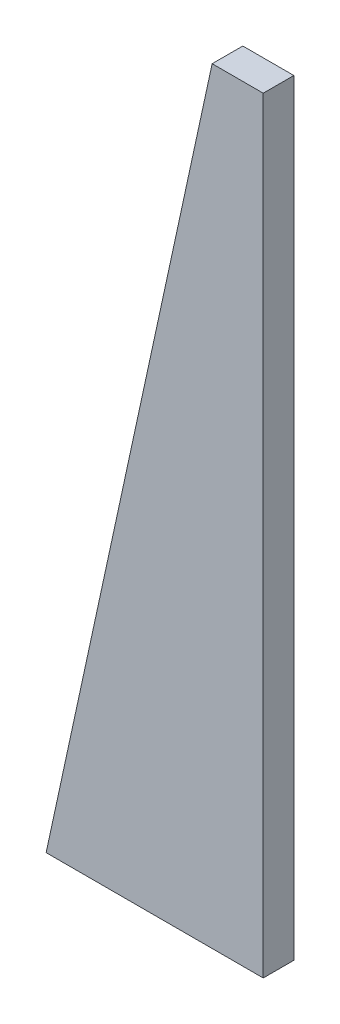
SolidWorks part; units mm, degrees
material "普通碳钢"
ref_plane "Front Plane" through (0, 0, 0) normal (0, 0, 1) x (1, 0, 0)
ref_plane "Top Plane" through (0, 0, 0) normal (0, 1, 0) x (1, 0, 0)
ref_plane "Right Plane" through (0, 0, 0) normal (1, 0, 0) x (0, 0, -1)
sketch "Sketch1" plane through (0, 0, 0) normal (0, 0, 1) x (1, 0, 0)
  line L0 (0, 0) -> (0, 300)
  line L1 (0, 0) -> (-85, 0)
  line L2 (0, 300) -> (-20, 300)
  line L3 (-20, 300) -> (-85, 0)
  dimension "D1" = 85
  dimension "D2" = 300
  dimension "D3" = 20
extrude "Extrude1" add sketch "Sketch1" along normal mid plane 12
